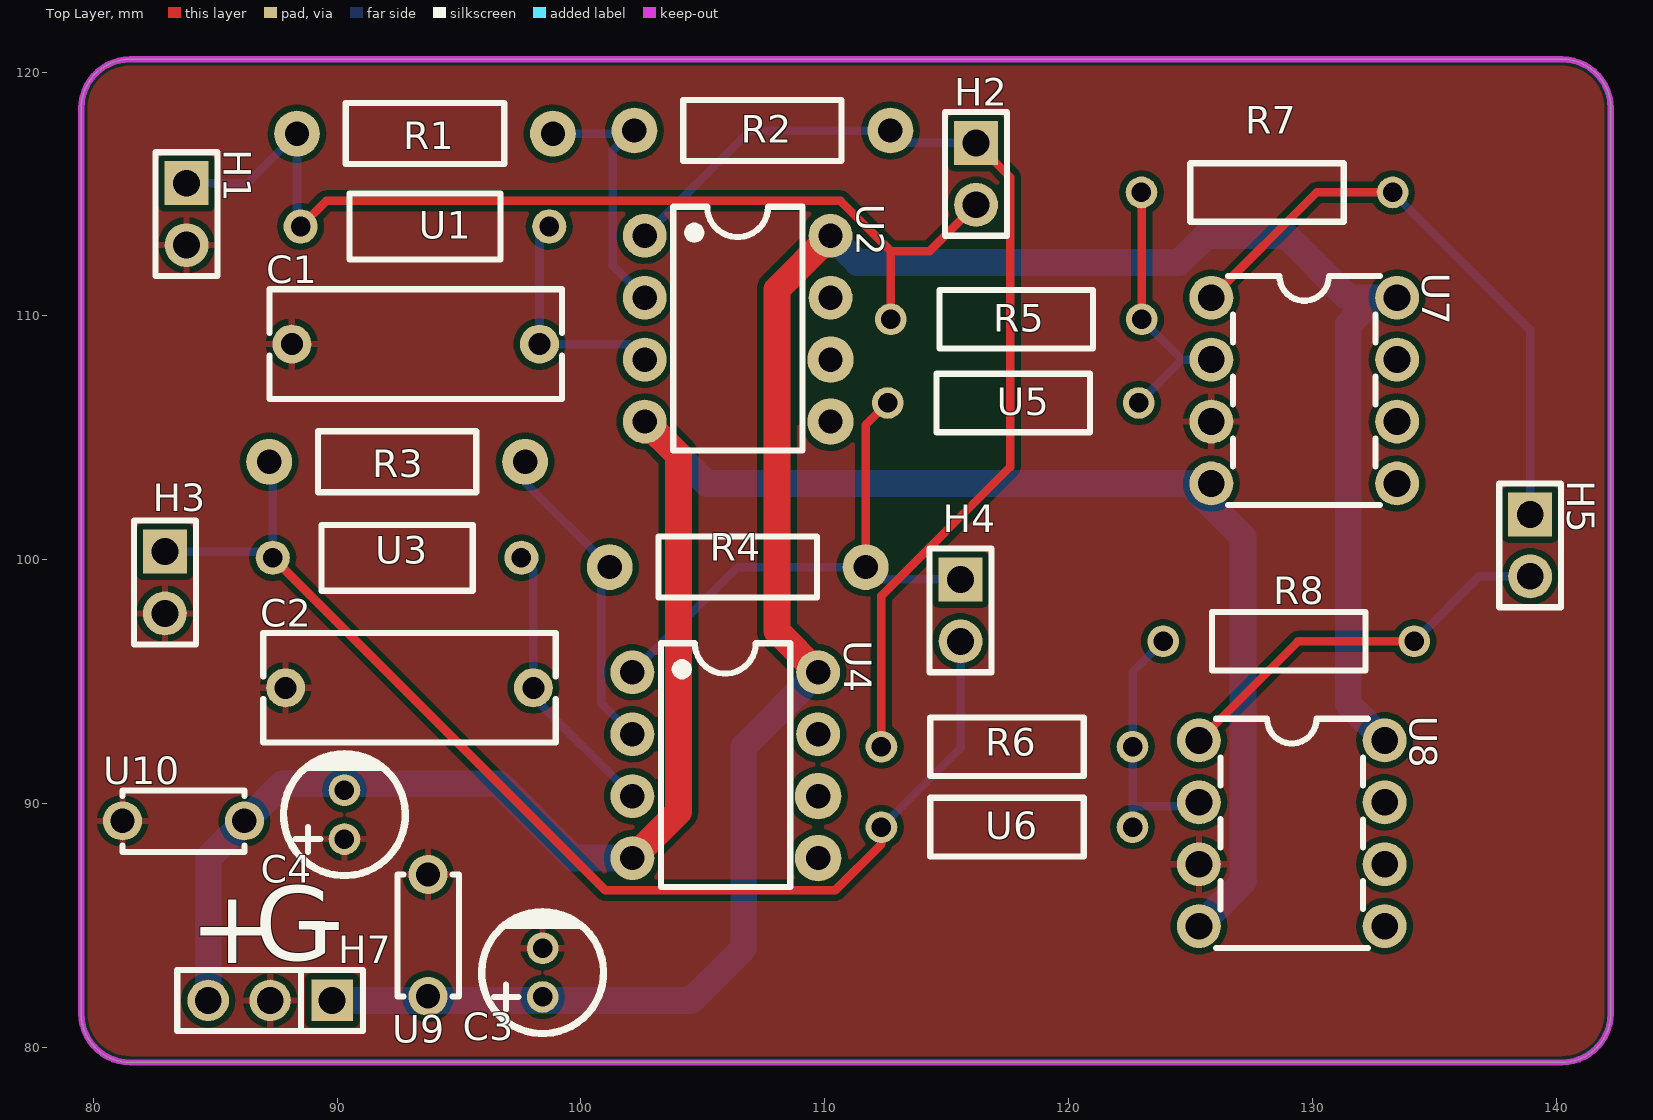
[diagram p0: Top Layer view]
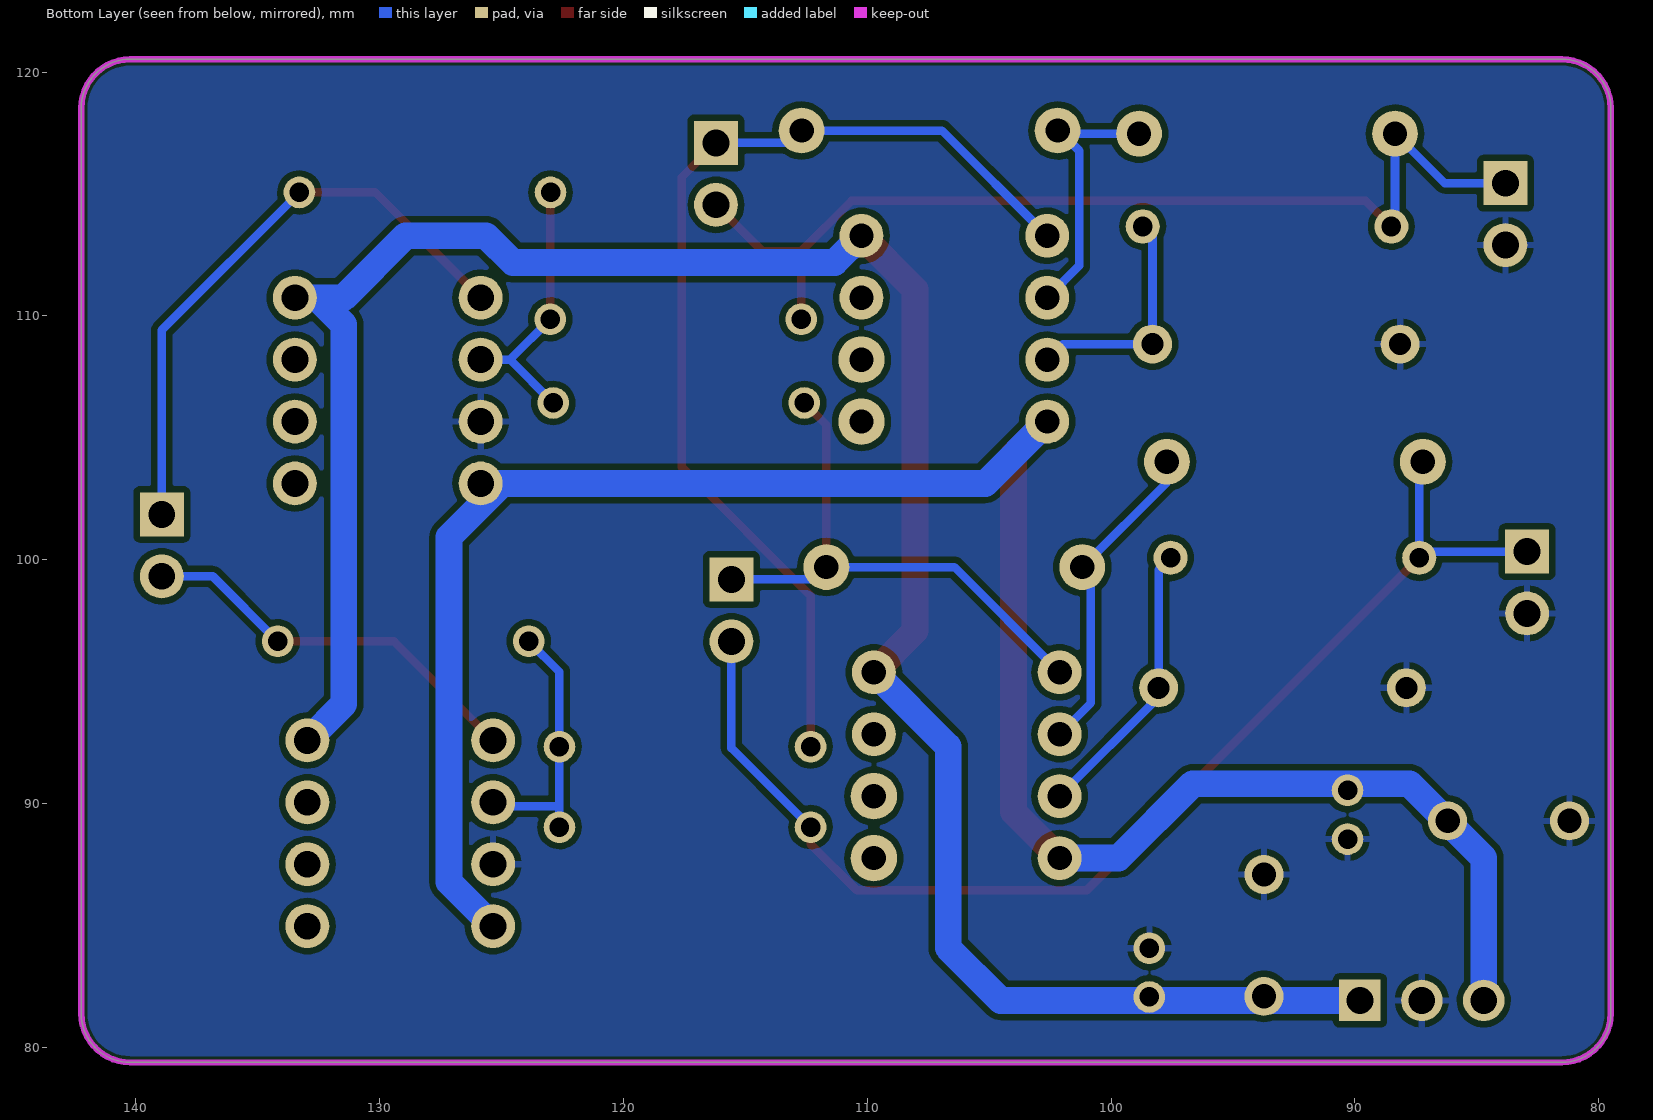
[diagram p1: Bottom Layer view, seen from below]
# Altium PCB MISC49900.pcbdoc
Units mm, origin at the board's own origin, x right, y up, seen from the top; angles counter-clockwise.
Board outline 62.74 x 41.15 mm, 2 copper layers (Top Layer, Bottom Layer), stack 1.58 mm thick; 28 components, 15 nets, 81 pads, 0 vias.

## Layer stack, top to bottom
Top Solder Mask Layer: solder mask 0.01, Dk 3.3
Top Layer: signal copper 0.035
Dielectric1: surface 1.51, FR4, Dk 4.5
Bottom Layer: signal copper 0.035
Bottom Solder Mask Layer: solder mask 0.01, Dk 3.3

## Board outline
81.502,120.523 ccw(c81.502,118.523) 79.502,118.523 79.502,81.375 ccw(c81.502,81.375) 81.502,79.375 140.24,79.375 ccw(c140.24,81.375) 142.24,81.375 142.24,118.523 ccw(c140.24,118.523) 140.24,120.523 81.502,120.523

## Design rules (kind name [scope] priority, off if disabled: settings)
BoardOutlineClearance copperThickness2oz_1 [All] p2 off: genericclearance=0.203 ignorepadtopadclearanceinfootprint=FALSE except(0: Arc-SplitContinuation Track-SplitContinuation SMDPad-SplitContinuation THPad-SplitContinuation Via-SplitContinuation Fill-SplitContinuation Region-SplitContinuation Poly-SplitContinuation Text-SplitContinuation Hole-SplitContinuation; 0.152: Arc-CutoutEdge SMDPad-CutoutEdge THPad-CutoutEdge Via-CutoutEdge Fill-CutoutEdge Region-CutoutEdge Text-CutoutEdge; 0.176: Hole-OutlineEdge Hole-CutoutEdge; 0.254: Poly-OutlineEdge Poly-CutoutEdge; 0.3: Arc-OutlineEdge Track-OutlineEdge SMDPad-OutlineEdge THPad-OutlineEdge Via-OutlineEdge Fill-OutlineEdge Region-OutlineEdge Text-OutlineEdge Track-CutoutEdge)
BoardOutlineClearance Plane_innerPlane_1 [All] p4 off: genericclearance=0.102 ignorepadtopadclearanceinfootprint=FALSE except(0: Arc-SplitContinuation Track-SplitContinuation SMDPad-SplitContinuation THPad-SplitContinuation Via-SplitContinuation Fill-SplitContinuation Region-SplitContinuation Poly-SplitContinuation Text-SplitContinuation Hole-SplitContinuation; 0.152: SMDPad-CutoutEdge THPad-CutoutEdge Via-CutoutEdge Fill-CutoutEdge Region-CutoutEdge Text-CutoutEdge; 0.176: Hole-OutlineEdge Hole-CutoutEdge; 0.254: Poly-OutlineEdge Poly-CutoutEdge; 0.3: Arc-OutlineEdge Track-OutlineEdge SMDPad-OutlineEdge THPad-OutlineEdge Via-OutlineEdge Fill-OutlineEdge Region-OutlineEdge Text-OutlineEdge Arc-CutoutEdge Track-CutoutEdge)
BoardOutlineClearance Copper_copperRegion_1 [All] p6 off: genericclearance=0.102 ignorepadtopadclearanceinfootprint=FALSE except(0: Arc-SplitContinuation Track-SplitContinuation SMDPad-SplitContinuation THPad-SplitContinuation Via-SplitContinuation Fill-SplitContinuation Region-SplitContinuation Poly-SplitContinuation Text-SplitContinuation Hole-SplitContinuation; 0.152: SMDPad-CutoutEdge THPad-CutoutEdge Via-CutoutEdge Fill-CutoutEdge Region-CutoutEdge Text-CutoutEdge; 0.176: Hole-OutlineEdge Hole-CutoutEdge; 0.254: Poly-OutlineEdge Poly-CutoutEdge; 0.3: Arc-OutlineEdge Track-OutlineEdge SMDPad-OutlineEdge THPad-OutlineEdge Via-OutlineEdge Fill-OutlineEdge Region-OutlineEdge Text-OutlineEdge Arc-CutoutEdge Track-CutoutEdge)
BoardOutlineClearance copperThickness1oz_1 [All] p8: genericclearance=0.102 ignorepadtopadclearanceinfootprint=FALSE except(0: Arc-SplitContinuation Track-SplitContinuation SMDPad-SplitContinuation THPad-SplitContinuation Via-SplitContinuation Fill-SplitContinuation Region-SplitContinuation Poly-SplitContinuation Text-SplitContinuation Hole-SplitContinuation; 0.152: SMDPad-CutoutEdge THPad-CutoutEdge Via-CutoutEdge Fill-CutoutEdge Region-CutoutEdge Text-CutoutEdge; 0.176: Hole-OutlineEdge Hole-CutoutEdge; 0.254: Poly-OutlineEdge Poly-CutoutEdge; 0.3: Arc-OutlineEdge Track-OutlineEdge SMDPad-OutlineEdge THPad-OutlineEdge Via-OutlineEdge Fill-OutlineEdge Region-OutlineEdge Text-OutlineEdge Arc-CutoutEdge Track-CutoutEdge)
Clearance copperThickness2oz [All] p1 off: gap=0.203 ignorepadtopadclearanceinfootprint=FALSE except(0.152: SMDPad-Track SMDPad-SMDPad THPad-Track SMDPad-THPad THPad-THPad Track-Via SMDPad-Via THPad-Via Via-Via Fill-Track Region-Track Fill-SMDPad Region-SMDPad Fill-THPad Region-THPad Fill-Via Region-Via Fill-Fill Fill-Region Region-Region Arc-Track Arc-SMDPad Arc-THPad Arc-Via Fill-Arc Region-Arc Arc-Arc Text-Track SMDPad-Text Text-THPad Text-Via Fill-Text Region-Text Arc-Text Text-Text; 0.176: Hole-Track Hole-SMDPad Hole-THPad Hole-Via Fill-Hole Region-Hole Hole-Arc Hole-Text; 0.254: Poly-Track Poly-SMDPad Poly-THPad Poly-Via Poly-Fill Poly-Region Poly-Poly Poly-Arc Poly-Text Poly-Hole)
Clearance Plane_innerPlane [All] p3 off: gap=0.102 ignorepadtopadclearanceinfootprint=FALSE except(0.152: SMDPad-Track SMDPad-SMDPad THPad-Track SMDPad-THPad THPad-THPad Track-Via SMDPad-Via THPad-Via Via-Via Fill-Track Region-Track Fill-SMDPad Region-SMDPad Fill-THPad Region-THPad Fill-Via Region-Via Fill-Fill Fill-Region Region-Region Arc-Track Arc-SMDPad Arc-THPad Arc-Via Fill-Arc Region-Arc Arc-Arc Text-Track SMDPad-Text Text-THPad Text-Via Fill-Text Region-Text Arc-Text Text-Text; 0.176: Hole-Track Hole-SMDPad Hole-THPad Hole-Via Fill-Hole Region-Hole Hole-Arc Hole-Text; 0.254: Poly-Track Poly-SMDPad Poly-THPad Poly-Via Poly-Fill Poly-Region Poly-Poly Poly-Arc Poly-Text Poly-Hole)
Clearance Copper_copperRegion [All] p5 off: gap=0.102 ignorepadtopadclearanceinfootprint=FALSE except(0.152: SMDPad-Track SMDPad-SMDPad THPad-Track SMDPad-THPad THPad-THPad Track-Via SMDPad-Via THPad-Via Via-Via Fill-Track Region-Track Fill-SMDPad Region-SMDPad Fill-THPad Region-THPad Fill-Via Region-Via Fill-Fill Fill-Region Region-Region Arc-Track Arc-SMDPad Arc-THPad Arc-Via Fill-Arc Region-Arc Arc-Arc Text-Track SMDPad-Text Text-THPad Text-Via Fill-Text Region-Text Arc-Text Text-Text; 0.176: Hole-Track Hole-SMDPad Hole-THPad Hole-Via Fill-Hole Region-Hole Hole-Arc Hole-Text; 0.254: Poly-Track Poly-SMDPad Poly-THPad Poly-Via Poly-Fill Poly-Region Poly-Poly Poly-Arc Poly-Text Poly-Hole)
Clearance copperThickness1oz [All] p7: gap=0.102 ignorepadtopadclearanceinfootprint=FALSE except(0.152: SMDPad-Track SMDPad-SMDPad THPad-Track SMDPad-THPad THPad-THPad Track-Via SMDPad-Via THPad-Via Via-Via Fill-Track Region-Track Fill-SMDPad Region-SMDPad Fill-THPad Region-THPad Fill-Via Region-Via Fill-Fill Fill-Region Region-Region Arc-Track Arc-SMDPad Arc-THPad Arc-Via Fill-Arc Region-Arc Arc-Arc Text-Track SMDPad-Text Text-THPad Text-Via Fill-Text Region-Text Arc-Text Text-Text; 0.176: Hole-Track Hole-SMDPad Hole-THPad Hole-Via Fill-Hole Region-Hole Hole-Arc Hole-Text; 0.254: Poly-Track Poly-SMDPad Poly-THPad Poly-Via Poly-Fill Poly-Region Poly-Poly Poly-Arc Poly-Text Poly-Hole)
DiffPairsRouting differentialPair [All] p1: maxlimit=0.152 minlimit=0.152 mostfreqgap=0.152 toplayer_minwidth=0.127 toplayer_prefwidth=0.254 toplayer_maxwidth=2.54 toplayer_mingap=0.152 toplayer_prefgap=0.152 toplayer_maxgap=0.152 bottomlayer_minwidth=0.127 bottomlayer_prefwidth=0.254 bottomlayer_maxwidth=2.54 bottomlayer_mingap=0.152 bottomlayer_prefgap=0.152 bottomlayer_maxgap=0.152 maxuncoupledlength=0.254
HoleToHoleClearance otherClearance [All] p1: gap=0.3 allowstackedmicrovias=TRUE
Length netLength [All] p1: minlimit=0 maxlimit=0
PasteMaskExpansion pasteMaskExpansion [All] p1: expansion=0
PlaneConnect innerPlane [All] p1: planeconnectstyle=Relief reliefexpansion=0.508 reliefentries=4 reliefconductorwidth=0.254 reliefairgap=0.254
PolygonConnect copperRegion [All] p1: connectstyle=Relief reliefconductorwidth=0.254 reliefentries=4 polygonreliefangle="90 Angle" airgapwidth=0.254 via.connectstyle=Relief via.reliefconductorwidth=0.254 via.reliefentries=4 via.polygonreliefangle="90 Angle" via.airgapwidth=0.254
RoutingVias viaSize [All] p1: holewidth=0.305 width=0.61 viastyle="Through Hole" minholewidth=0.3 minwidth=0.5 maxholewidth=6.3 maxwidth=10
SolderMaskExpansion solderMaskExpansion [IsVia] p1: expansion=-25.4 istentingtop=TRUE
SolderMaskExpansion solderMaskExpansion [All] p2: expansion=0.051 istentingtop=FALSE
Width copperThickness2oz_2 [(InNet('+15V') OR InNet('-15V'))] p1: maxlimit=2.54 minlimit=0.203 preferedwidth=1.1
Width copperThickness1oz_2 [All] p2: maxlimit=2.54 minlimit=0.127 preferedwidth=0.351

## Components (designator, comment, footprint, x,y, rotation, side; value= is the part's Value field where it differs from the comment)
C1 "22nF" CAP-TH_L12.0-W4.5-P10.00-D1.0 93.218,108.839 r0 top
C2 "22nF" CAP-TH_L12.0-W4.5-P10.00-D1.0 92.964,94.742 r0 top
C3 "10uF" CAP-TH_BD5.0-P2.00-D0.8-FD-10UF50VC110GL 98.425,83.058 r90 top
C4 "10uF" CAP-TH_BD5.0-P2.00-D0.8-FD-10UF50VC110GL 90.297,89.535 r90 top
H1 "" HDR-TH_2P-P2.54-V-M-1 83.82,114.173 r270 top
H2 "" HDR-TH_2P-P2.54-V-M-1 116.205,115.824 r270 top
H3 "" HDR-TH_2P-P2.54-V-M-1 82.931,99.06 r270 top
H4 "" HDR-TH_2P-P2.54-V-M-1 115.57,97.917 r270 top
H5 "" HDR-TH_2P-P2.54-V-M-1 138.938,100.584 r270 top
H7 "" HDR-TH_3P-P2.54-V-M 87.249,81.915 r180 top
R1 "1kΩ" RES-TH_BD2.5-L6.5-P10.50-D0.6 93.599,117.475 r0 top
R2 "1kΩ" RES-TH_BD2.5-L6.5-P10.50-D0.6 107.442,117.602 r0 top
R3 "1kΩ" RES-TH_BD2.5-L6.5-P10.50-D0.6 92.456,104.013 r0 top
R4 "1kΩ" RES-TH_BD2.5-L6.5-P10.50-D0.6 106.426,99.695 r0 top
R5 "20kΩ" RES-TH_BD2.4-L6.3-P10.30-D0.6 117.856,109.855 r0 top
R6 "20kΩ" RES-TH_BD2.4-L6.3-P10.30-D0.6 117.475,92.329 r0 top
R7 "20kΩ" RES-TH_BD2.4-L6.3-P10.30-D0.6 128.143,115.062 r0 top
R8 "20kΩ" RES-TH_BD2.4-L6.3-P10.30-D0.6 129.032,96.647 r0 top
U1 "8.2kΩ" RES-TH_BD2.7-L6.2-P10.20-D0.4 93.599,113.665 r0 top
U2 "LF353N/NOPB" PDIP-8_L9.6-W6.4-P2.54-LS7.6-BL 106.426,109.474 r270 top
U3 "8.2kΩ" RES-TH_BD2.7-L6.2-P10.20-D0.4 92.456,100.076 r0 top
U4 "LF353N/NOPB" PDIP-8_L9.6-W6.4-P2.54-LS7.6-BL 105.918,91.567 r270 top
U5 "39kΩ" RES-TH_BD2.4-L6.3-P10.30-D0.6 117.729,106.426 r0 top
U6 "39kΩ" RES-TH_BD2.4-L6.3-P10.30-D0.6 117.475,89.027 r0 top
U7 "LM358N(XBLW)" PDIP-8_L9.3-W6.4-P2.54-LS7.6-BL 129.667,106.934 r270 top
U8 "LM358N(XBLW)" PDIP-8_L9.3-W6.4-P2.54-LS7.6-BL 129.159,88.773 r270 top
U9 "100nF" CAP-TH_L5.0-W2.5-P5.00-D1.0 93.726,84.582 r90 top
U10 "100nF" CAP-TH_L5.0-W2.5-P5.00-D1.0 83.693,89.281 r0 top

## Footprints (in the part's own frame and the unit in brackets; to place one, negate y for a bottom-side part, rotate by r counter-clockwise, add the part's x,y. Pads: shape width x height; smd on the part's side, far side on the other; paste and mask are expansions set on the pad)
CAP-TH_BD5.0-P2.00-D0.8-FD-10UF50VC110GL [mm]
  round 1.3 hole 0.8: 1(-1,0) 2(1,0)
  silkscreen extent -2.5,-2.5 2.5,2.5
CAP-TH_L5.0-W2.5-P5.00-D1.0 [mm]
  round 1.6 hole 1: 1(-2.5,0) 2(2.5,0)
  silkscreen extent -2.5,-1.27 2.5,1.25
CAP-TH_L12.0-W4.5-P10.00-D1.0 [mm]
  round 1.6 hole 0.9: 1(-5.08,0) 2(5.08,0)
  silkscreen extent -6,-2.25 6,2.25
HDR-TH_2P-P2.54-V-M-1 [mm]
  rect 1.8x1.8 hole 1.1: 1(-1.27,0)
  round 1.8 hole 1.1: 2(1.27,0)
  silkscreen extent -2.54,-1.27 2.54,1.27
HDR-TH_3P-P2.54-V-M [mm]
  rect 1.7x1.7 hole 1.1: 1(-2.54,0)
  round 1.7 hole 1.1: 2(0,0) 3(2.54,0)
  silkscreen extent -3.81,-1.25 3.81,1.25
PDIP-8_L9.3-W6.4-P2.54-LS7.6-BL [mm]
  round 1.8 hole 1.1: 1(-3.81,-3.81) 2(-1.27,-3.81) 3(1.27,-3.81) 4(3.81,-3.81) 5(3.81,3.81) 6(1.27,3.81) 7(-1.27,3.81) 8(-3.81,3.81)
  silkscreen extent -4.7,-3.11 4.7,3.11
PDIP-8_L9.6-W6.4-P2.54-LS7.6-BL [mm]
  round 1.8 hole 1: 1(-3.81,-3.81) 2(-1.27,-3.81) 3(1.27,-3.81) 4(3.81,-3.81) 7(-1.27,3.81) 8(-3.81,3.81)
  round 1.905 hole 1: 5(3.81,3.81) 6(1.27,3.81)
  silkscreen extent -5,-2.64 5,2.67
RES-TH_BD2.4-L6.3-P10.30-D0.6 [mm]
  round 1.3 hole 0.8: 1(-5.15,0) 2(5.15,0)
  silkscreen extent -3.15,-1.2 3.15,1.2
RES-TH_BD2.5-L6.5-P10.50-D0.6 [mm]
  round 1.88 hole 1: 1(-5.25,0) 2(5.25,0)
  silkscreen extent -3.25,-1.25 3.25,1.25
RES-TH_BD2.7-L6.2-P10.20-D0.4 [mm]
  round 1.4 hole 0.8 copper offset 0,0: 1(-5.1,0) 2(5.1,0)
  silkscreen extent -3.1,-1.35 3.1,1.35

## Nets (pads, with @x,y where several pads share a name; then routed paths per layer and width w, separated by ;. In a path a pad name is that pad's centre, name@x,y a point inside that pad or via, vN(x,y) a via of type N, cw(c..) or ccw(c..) an arc to the next point about the centre after c; other vN are vias at no path point)
$1N2: H1.1 H2.2 R1.1 R5.1 U1.1 | length 41.8
  Top Layer w0.35: U1.1 89.549,114.715 110.646,114.715 112.706,112.655 ; R5.1 112.706,112.655 ; H2.2 114.306,112.655 112.706,112.655
  Bottom Layer w0.35: H1.1 86.317,115.443 R1.1 88.349,113.815 U1.1
$1N3: R1.2 R2.1 U2.2 | length 11
  Bottom Layer w0.35: R1.2 R2.1@101.999,117.475 ; R2.1 102.065,117.475 R2.1@101.999,117.475 ; U2.2 101.299,112.061 101.299,116.775 R2.1@101.999,117.475
$1N5: C1.2 U1.2 U2.3 | length 9.6
  Bottom Layer w0.35: U1.2 98.298,113.264 C1.2 101.981,108.839 U2.3
$1N9: H2.1 R2.2 R6.1 U2.1 | length 43.1
  Top Layer w0.35: R6.1 112.325,98.514 117.605,103.794 117.605,115.694 H2.1
  Bottom Layer w0.35: U2.1 106.934,117.602 R2.2 113.2,117.094 H2.1
$1N10: H4.1 R4.2 U4.1 U5.1 | length 22.6
  Top Layer w0.35: R4.2 111.676,105.523 U5.1
  Bottom Layer w0.35: U4.1 106.426,99.695 R4.2 112.184,99.187 H4.1
$1N14: C2.2 U3.2 U4.3 | length 11.7
  Bottom Layer w0.35: U3.2 98.044,99.588 C2.2 98.044,94.361 U4.3
$1N15: R3.2 R4.1 U4.2 | length 13.3
  Bottom Layer w0.35: R3.2 97.706,103.165 R4.1 100.826,99.345 100.826,94.119 U4.2
$1N16: H3.1 H4.2 R3.1 U3.1 U6.1 | length 49.6
  Top Layer w0.35: U3.1 100.997,86.435 110.433,86.435 112.325,88.327 U6.1
  Bottom Layer w0.35: H3.1 87.102,100.33 U3.1 87.356,103.863 R3.1 ; U6.1 115.57,92.272 H4.2
$1N18: R5.2 R7.1 U5.2 U7.2 | length 11.3
  Top Layer w0.35: R7.1 123.006,115.049 R5.2
  Bottom Layer w0.35: U5.2 124.657,108.204 ; R5.2 124.657,108.204 ; U7.2 124.657,108.204
$1N19: R6.2 R8.1 U6.2 U8.2 | length 10.9
  Bottom Layer w0.35: U6.2 122.625,89.879 ; R8.1 122.625,95.39 R6.2 122.625,89.879 ; U8.2 125.185,89.879 122.625,89.879
$1N23: H5.1 R7.2 U7.1 | length 24.8
  Top Layer w0.35: U7.1 130.175,115.062 R7.2
  Bottom Layer w0.35: R7.2 138.938,109.417 H5.1
$1N24: H5.2 R8.2 U8.1 | length 16.4
  Top Layer w0.35: U8.1 129.413,96.647 R8.2
  Bottom Layer w0.35: R8.2 136.849,99.314 H5.2
+15V: C3.1 H7.1 U2.8 U4.8 U7.8 U8.8 U9.1 | length 94.3
  Top Layer w1.1: U4.8 108.036,97.069 108.036,111.084 U2.8
  Bottom Layer w1.1: H7.1 104.521,81.915 106.68,84.074 106.68,92.329 U4.8 ; U2.8 111.336,112.184 124.536,112.184 125.636,113.284 128.936,113.284 131.476,110.744 132.576,110.744 ; U8.8 131.476,94.076 131.476,109.644 132.576,110.744 ; U7.8 132.576,110.744
-15V: C4.2 H7.3 U2.4 U4.4 U7.4 U8.4 U10.2 | length 89.1
  Top Layer w1.1: U4.4 103.994,89.643 103.994,104.286 U2.4
  Bottom Layer w1.1: H7.3 84.709,87.757 87.757,90.805 96.647,90.805 99.695,87.757 U4.4 ; U2.4 105.156,103.124 124.956,103.124 ; U8.4 127.156,86.77 127.156,100.924 124.956,103.124 ; U7.4 124.956,103.124
GND: C1.1 C2.1 C3.2 C4.1 H1.2 H3.2 H7.2 U7.3 U8.3 U9.2 U10.1
pads on no net: U2.5 U2.6 U2.7 U4.5 U4.6 U4.7 U7.5 U7.6 U7.7 U8.5 U8.6 U8.7

## Polygon pours and split planes (outlines as drawn)
GND on Top Layer (solid, remove dead copper, pour order 0): 76.2,122.555 76.2,77.089 144.526,77.089 144.526,122.555
GND on Bottom Layer (solid, remove dead copper, pour order 2): 78.232,122.428 78.232,76.2 147.828,76.2 147.828,122.428

## Keep-outs
Board Outline Layer:
  the board outline again, w0.254

## Silkscreen, mask and mechanical layers (free items; w line width, h text height)
Top Silkscreen Layer:
  text "-" at 88.773,83.82 h3.05
  text "G" at 86.614,83.566 h3.05
  text "+" at 83.947,83.439 h3.05